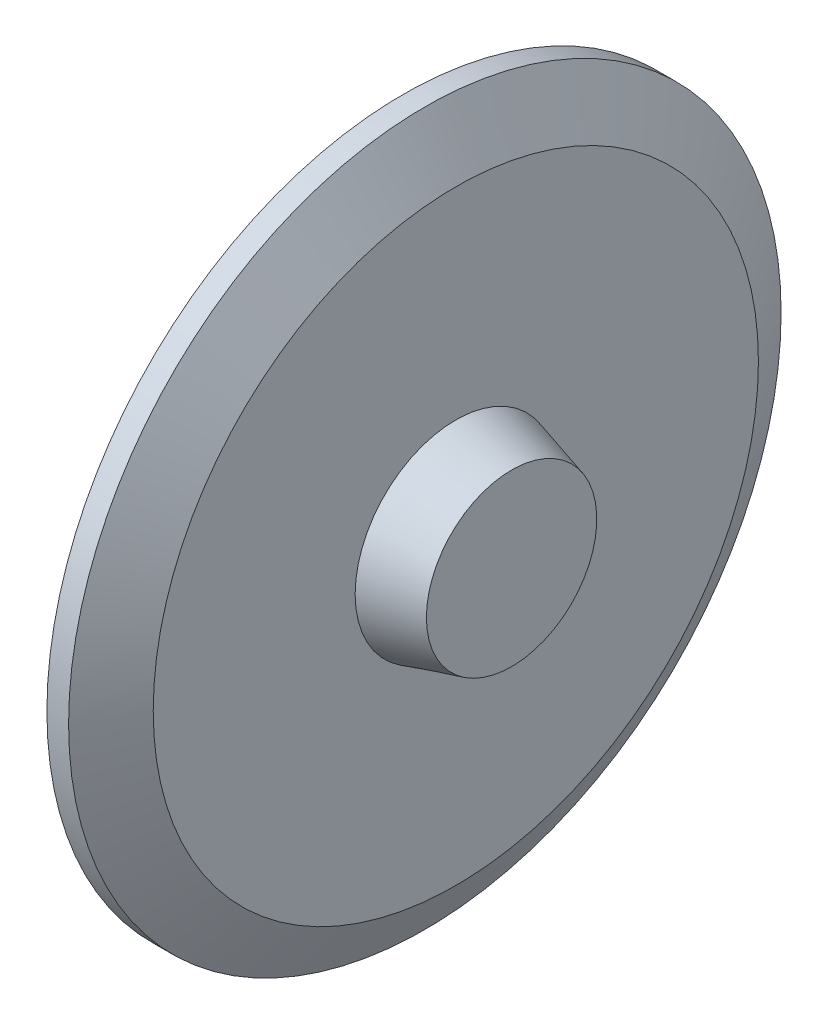
from build123d import *


with BuildPart() as part:
    # Sketch1 → Revolve1 (revolve)
    with BuildSketch(Plane.XY, mode=Mode.PRIVATE) as revolve1_sk:
        Polygon((0, 0), (0, 100), (4, 100), (4, 115), (11, 115), (21, 97.679491924), (21, 32.5), (39, 27.5), (39, 0), align=None)
    revolve(revolve1_sk.sketch.rotate(Axis((0, 0, 0), (1, 0, 0)), 90), axis=Axis((0, 0, 0), (1, 0, 0)))


solid = part.part
